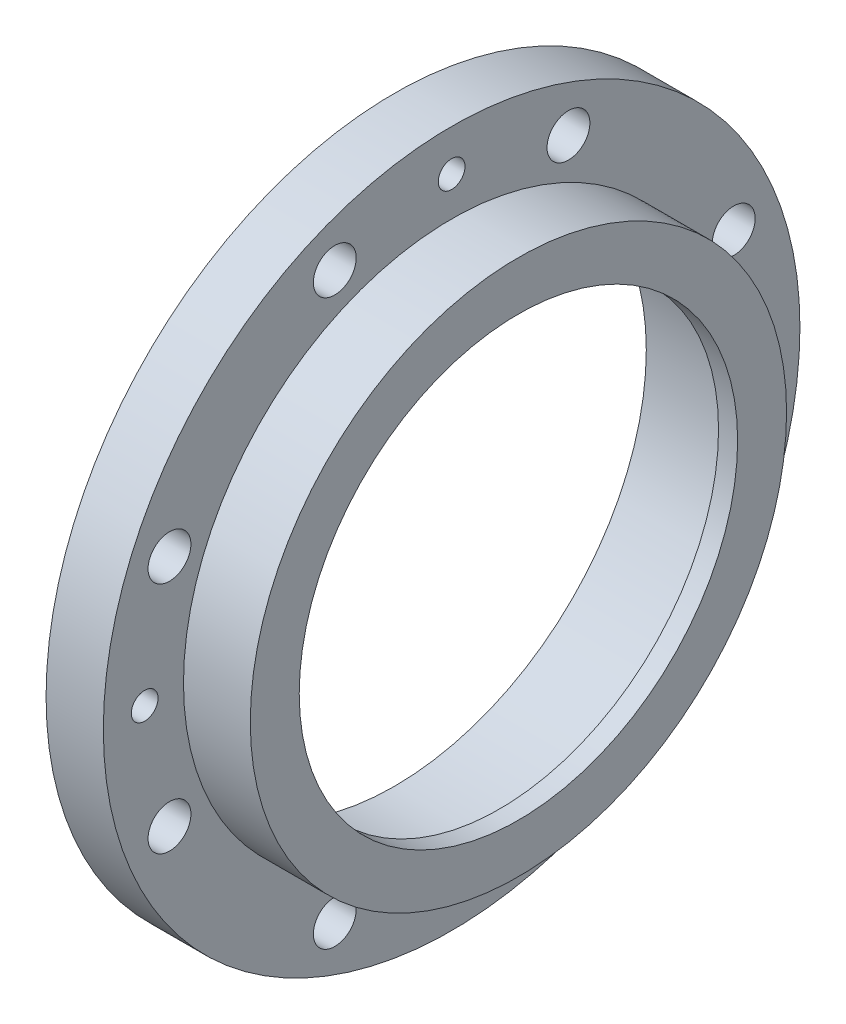
from build123d import *

# Parameters (mm, degrees)
SKETCH2_R          = 11.22654111
CUT_EXTRUDE1_DEPTH = 30
CIRPATTERN1_COUNT  = 4


with BuildPart() as part:
    # Sketch1 → Revolve1 (revolve)
    with BuildSketch(Plane.XY, mode=Mode.PRIVATE) as revolve1_sk:
        Polygon((-79.177234861, 132), (-79.177234861, 182.5), (-49.177234861, 182.5), (-49.177234861, 140.5), (-14.177234861, 140.5), (-14.177234861, 114.860017889), (-24.177234861, 114.860017889), (-24.177234861, 132), align=None)
    revolve(revolve1_sk.sketch.rotate(Axis((-169.440966011, 0, 0), (1, 0, 0)), 90), axis=Axis((-169.440966011, 0, 0), (1, 0, 0)))

    # Sketch2 → Cut-Extrude1 (cut)
    with BuildSketch(Plane.ZY.offset(79.177234861)):
        with Locations((61.229349178, 147.820725202)):
            Circle(SKETCH2_R)
        with Locations((147.820725202, 61.229349178)):
            Circle(SKETCH2_R)
        with Locations((147.820725202, -61.229349178)):
            Circle(SKETCH2_R)
        with Locations((61.229349178, -147.820725202)):
            Circle(SKETCH2_R)
        with Locations((-61.229349178, -147.820725202)):
            Circle(SKETCH2_R)
        with Locations((-147.820725202, -61.229349178)):
            Circle(SKETCH2_R)
        with Locations((-147.820725202, 61.229349178)):
            Circle(SKETCH2_R)
        with Locations((-61.229349178, 147.820725202)):
            Circle(SKETCH2_R)
    extrude(amount=-CUT_EXTRUDE1_DEPTH, mode=Mode.SUBTRACT)

    # Sketch6 → M16 Tapped Hole1 (revolve, cut)
    with BuildSketch(Plane(origin=(-79.177234861, 160.836236417, 0), x_dir=(0, 0, 1), z_dir=(0, 1, 0))):
        Polygon((0, 0), (0, 46.206024333), (7, 42), (7, 0), align=None)
    m16_tapped_hole1 = revolve(axis=Axis((-85.527234861, 160.836236417, 0), (1, 0, 0)), mode=Mode.SUBTRACT)

    # CirPattern1: M16 Tapped Hole1 ×4 about axis
    cirpattern1_axis = Axis((0, 0, 0), (1, 0, 0))
    for i in range(1, CIRPATTERN1_COUNT):
        add(m16_tapped_hole1.rotate(cirpattern1_axis, i * 360 / CIRPATTERN1_COUNT), mode=Mode.SUBTRACT)


solid = part.part
